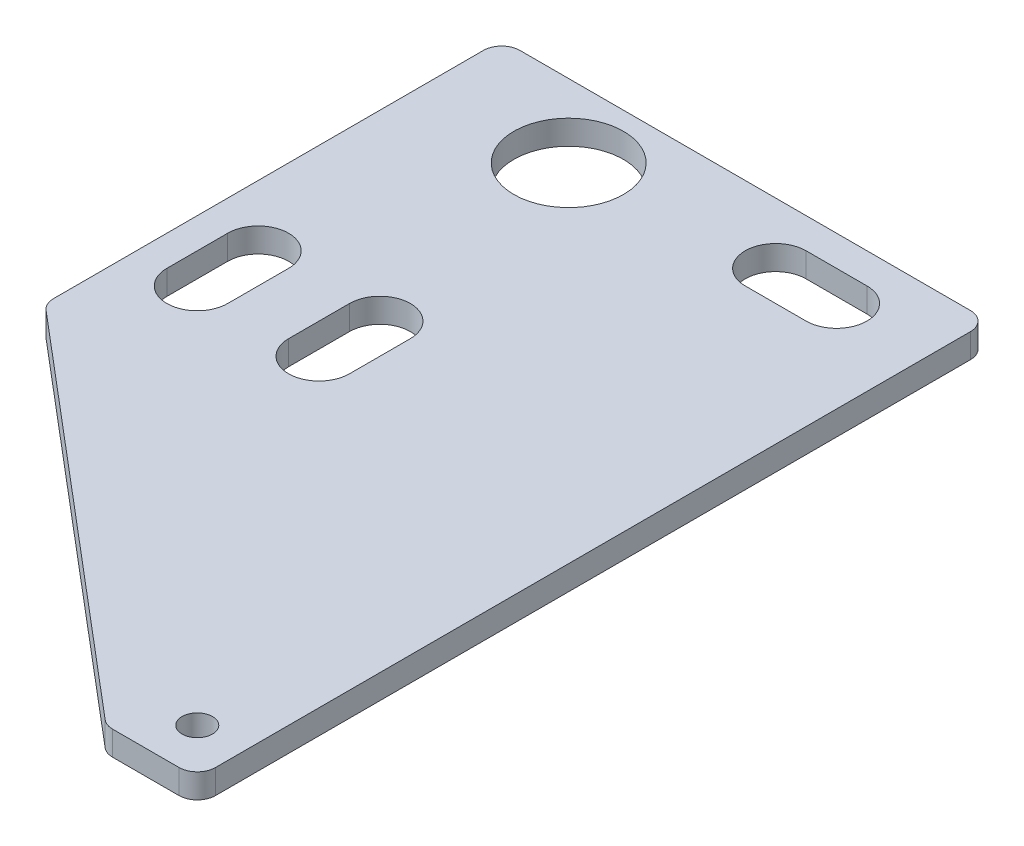
SolidWorks part; units mm, degrees
material "SPCC"
ref_plane "Front" through (0, 0, 0) normal (0, 0, 1) x (1, 0, 0)
ref_plane "Top" through (0, 0, 0) normal (0, 1, 0) x (1, 0, 0)
ref_plane "Right" through (0, 0, 0) normal (1, 0, 0) x (0, 0, -1)
sketch "Sketch1" plane through (0, 0, 0) normal (0, 1, 0) x (1, 0, 0)
  line L0 (0, 0) -> (-80, 0)
  line L1 (-80, 0) -> (-80, -75)
  line L3 (-15, -130) -> (0, -130)
  line L4 (0, -130) -> (0, 0)
  line L5 (-25, -10) -> (-15, -10) construction
  line L6 (-25, -5) -> (-15, -5)
  line L7 (-25, -15) -> (-15, -15)
  line L8 (-70, -50) -> (-70, -60) construction
  line L9 (-65, -50) -> (-65, -60)
  line L10 (-75, -50) -> (-75, -60)
  line L11 (-50, -50) -> (-50, -60) construction
  line L12 (-45, -50) -> (-45, -60)
  line L13 (-55, -50) -> (-55, -60)
  line L14 (-80, -75) -> (-15, -130)
  circle A0 centre (-57, -12) radius 9
  arc A1 (-25, -5) -> (-25, -15) centre (-25, -10) ccw
  arc A2 (-15, -15) -> (-15, -5) centre (-15, -10) ccw
  arc A3 (-65, -50) -> (-75, -50) centre (-70, -50) ccw
  arc A4 (-75, -60) -> (-65, -60) centre (-70, -60) ccw
  arc A5 (-45, -50) -> (-55, -50) centre (-50, -50) ccw
  arc A6 (-55, -60) -> (-45, -60) centre (-50, -60) ccw
  circle A7 centre (-7.5, -122.5) radius 2.5
  point P10 (-20, -10)
  point P17 (-70, -55)
  point P22 (-50, -55)
  dimension "D5" = 18
  dimension "D11" = 57
  dimension "D18" = 5
  dimension "D19" = 7.5
  dimension "D20" = 7.5
  dimension "D1" = 80
  dimension "D2" = 75
  dimension "D3" = 130
  dimension "D4" = 15
  dimension "D6" = 10
  dimension "D7" = 15
  dimension "D8" = 10
  dimension "D9" = 10
  dimension "D10" = 12
  dimension "D12" = 10
  dimension "D13" = 10
  dimension "D14" = 10
  dimension "D15" = 50
  dimension "D16" = 20
  dimension "D17" = 50
extrude "Boss-Extrude1" add sketch "Sketch1" along normal blind 4
fillet "Fillet1" radius 3 5 edges at (-15, 2, 130) (-80, 2, 75) (-80, 2, 0) (0, 2, 0) (0, 2, 130)
sketch "Sketch2" plane through (0, 0, 0) normal (0, -1, 0) x (1, 0, 0)
  circle A0 centre (-70, 50) radius 5
  circle A1 centre (-50, 50) radius 5
surface "Surface-Extrude1" [suppressed] sketch "Sketch2"
